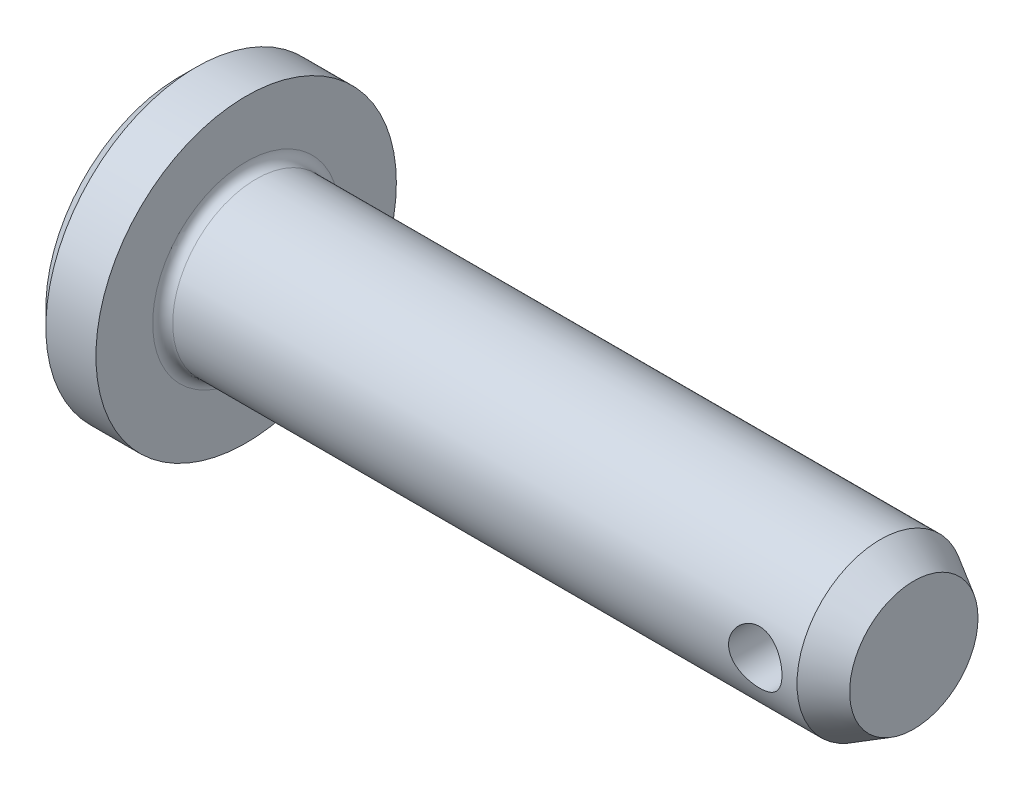
SolidWorks part; units mm, degrees
material "Q235"
ref_plane "Front" through (0, 0, 0) normal (0, 0, 1) x (1, 0, 0)
ref_plane "Top" through (0, 0, 0) normal (0, 1, 0) x (1, 0, 0)
ref_plane "Right" through (0, 0, 0) normal (1, 0, 0) x (0, 0, -1)
sketch "Dimension sketch" plane through (0, 0, 0) normal (0, 0, 1) x (1, 0, 0)
  line L0 (0, 18) -> (0, 0)
  line L1 (0, 0) -> (40, 0)
  circle A0 centre (35.5, 0) radius 1.6 construction
  point P3 (0, 10)
  point P5 (4, 0)
  point P6 (0.6, 0)
  point P7 (38, 0)
  point P8 (5, 0)
  dimension "d1" = 3.2
  dimension "l" = 40
  dimension "dk" = 18
  dimension "d" = 10
  dimension "k" = 4
  dimension "r" = 0.6
  dimension "c" = 2
  dimension "e" = 1
  dimension "le" = 4.5
sketch "Sketch1" plane through (0, 0, 0) normal (0, 0, 1) x (1, 0, 0)
  line L0 (0, 0) -> (-7.3443, 0) construction
  line L1 (0, 0) -> (44, 0)
  line L2 (0, 0) -> (0, 8)
  line L3 (1, 9) -> (4, 9)
  line L4 (4, 9) -> (4, 5)
  line L5 (4, 5) -> (44, 5)
  line L6 (44, 5) -> (44, 0)
  line L7 (0, 8) -> (1, 9)
  point P4 (0, 9)
  dimension "D2" = 18
  dimension "D1" = 40
  dimension "D3" = 10
  dimension "D4" = 4
revolve "Base-Revolve" add sketch "Sketch1" angle 360 about L0
sketch "Sketch2" plane through (0, 0, 0) normal (0, 0, 1) x (1, 0, 0)
  line L0 (0, 0) -> (40, 0) construction
  line L1 (44, -5) -> (44, 5) construction
  circle A1 centre (39.5, 0) radius 1.6
  dimension "D1" = 3.2
  dimension "D2" = 4.5
extrude "Cut-Extrude1" cut sketch "Sketch2" against normal through all and the other way through all
fillet "Fillet1" radius 0.6 1 edges at (4, 0, -5)
chamfer "Chamfer1" distance 2 angle 30 1 edges at (44, 0, -5)
